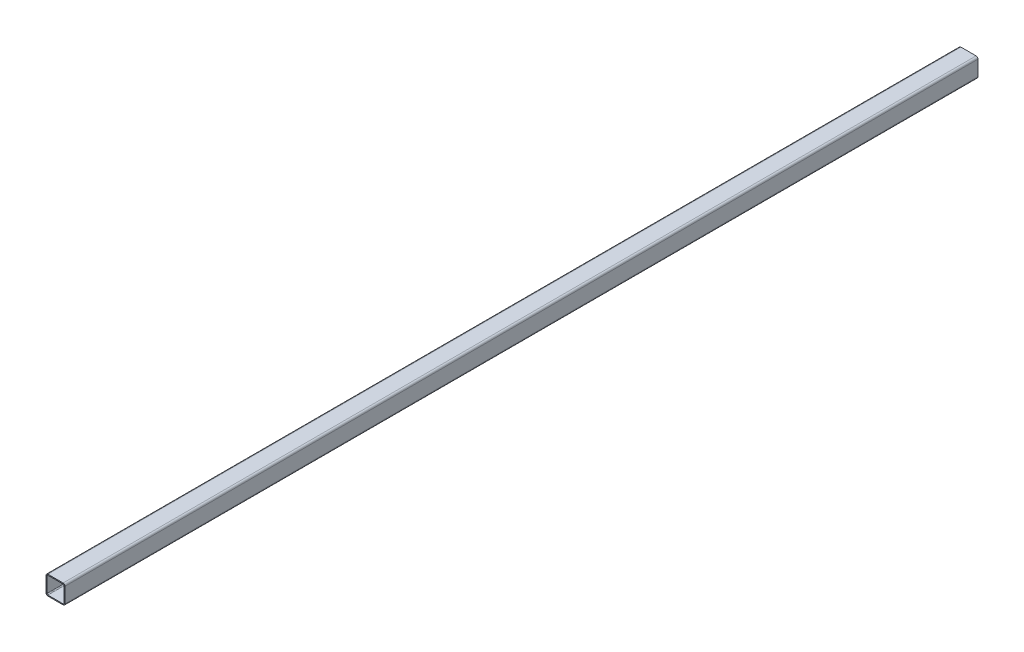
from build123d import *

# Parameters (mm, degrees)
BOSS_EXTRUDE_1_DEPTH = 2400


with BuildPart() as part:
    # Sketch 1 → Boss-Extrude 1 (new, symmetric)
    with BuildSketch(Plane.XY):
        with BuildLine():
            Line((0, 50), (-40, 50))
            ThreePointArc((-40, 50), (-47.071067812, 47.071067812), (-50, 40))
            Line((-50, 40), (-50, 0))
            Line((-50, 0), (-50, -40))
            ThreePointArc((-50, -40), (-47.071067812, -47.071067812), (-40, -50))
            Line((-40, -50), (40, -50))
            ThreePointArc((40, -50), (47.071067812, -47.071067812), (50, -40))
            Line((50, -40), (50, 0))
            Line((50, 0), (50, 40))
            ThreePointArc((50, 40), (47.071067812, 47.071067812), (40, 50))
            Line((40, 50), (0, 50))
        make_face()
        with BuildLine():
            Line((0, 45), (-40, 45))
            ThreePointArc((-40, 45), (-43.535533906, 43.535533906), (-45, 40))
            Line((-45, 40), (-45, 0))
            Line((-45, 0), (-45, -40))
            ThreePointArc((-45, -40), (-43.535533906, -43.535533906), (-40, -45))
            Line((-40, -45), (40, -45))
            ThreePointArc((40, -45), (43.535533906, -43.535533906), (45, -40))
            Line((45, -40), (45, 0))
            Line((45, 0), (45, 40))
            ThreePointArc((45, 40), (43.535533906, 43.535533906), (40, 45))
            Line((40, 45), (0, 45))
        make_face(mode=Mode.SUBTRACT)
    extrude(amount=BOSS_EXTRUDE_1_DEPTH, both=True)


solid = part.part
